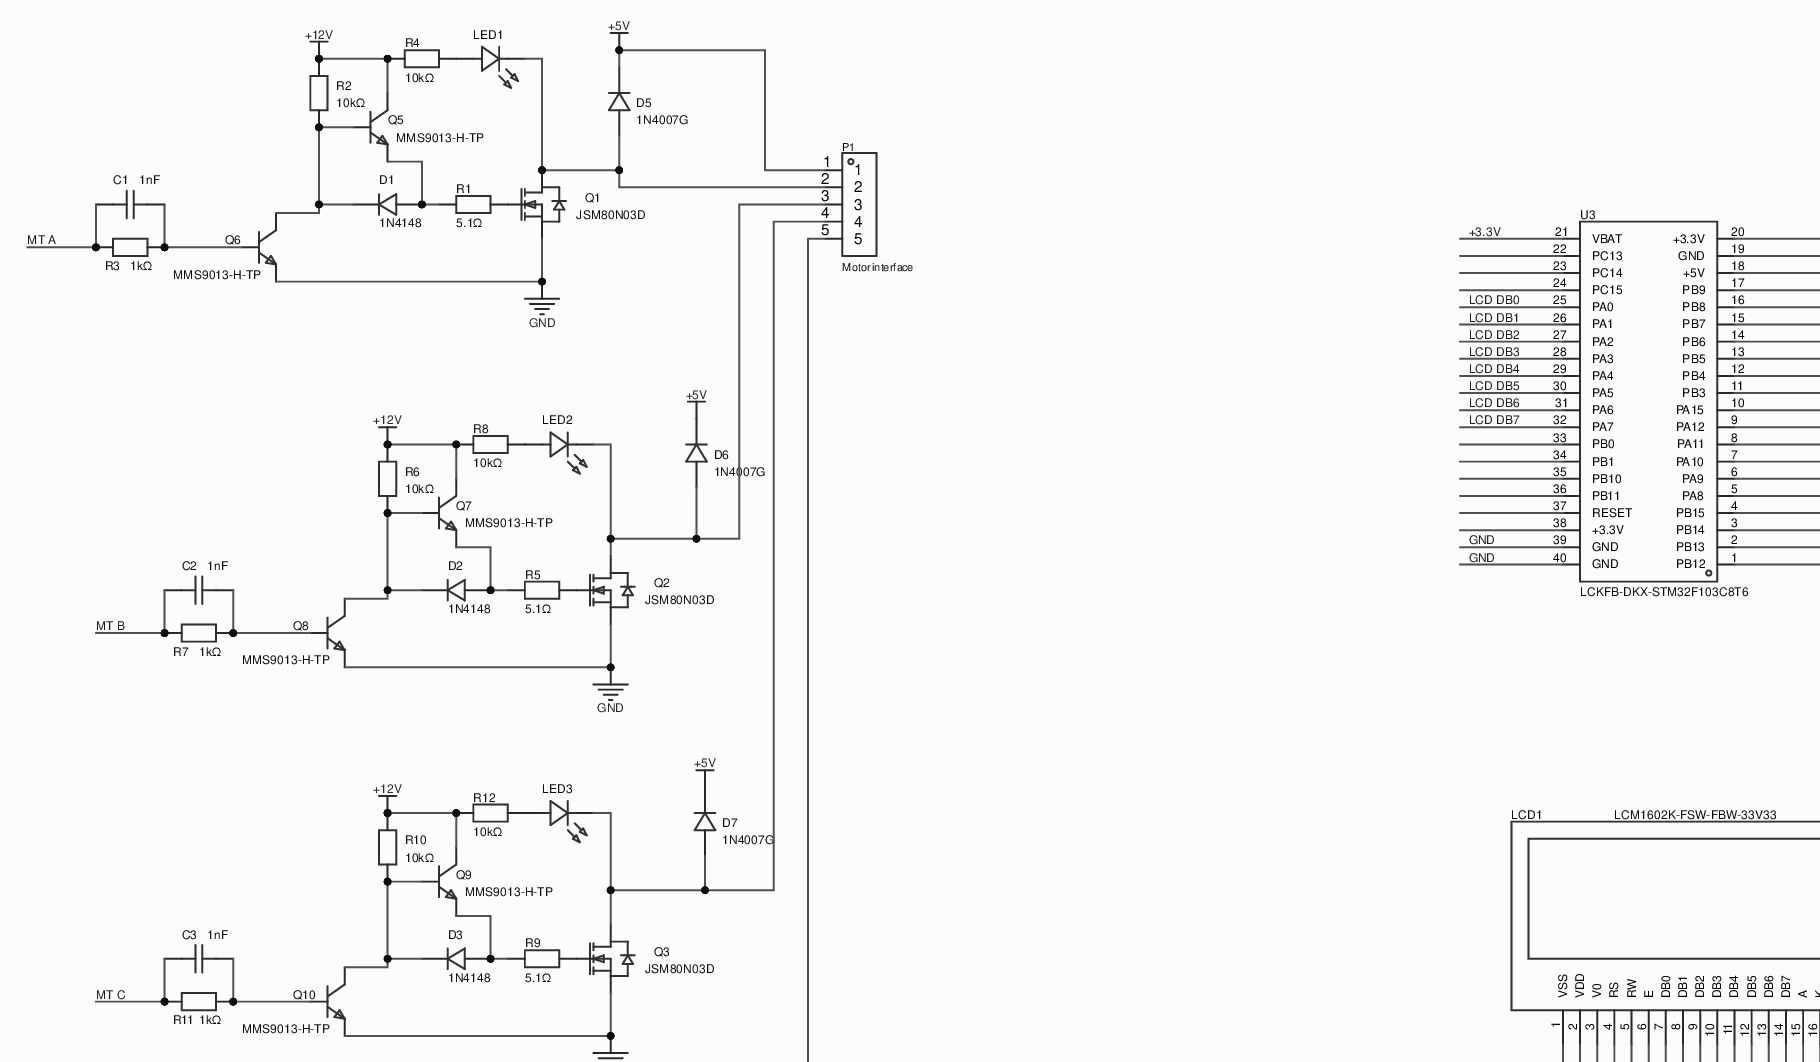
[diagram p0: MISC49935-3.schdoc, top left]
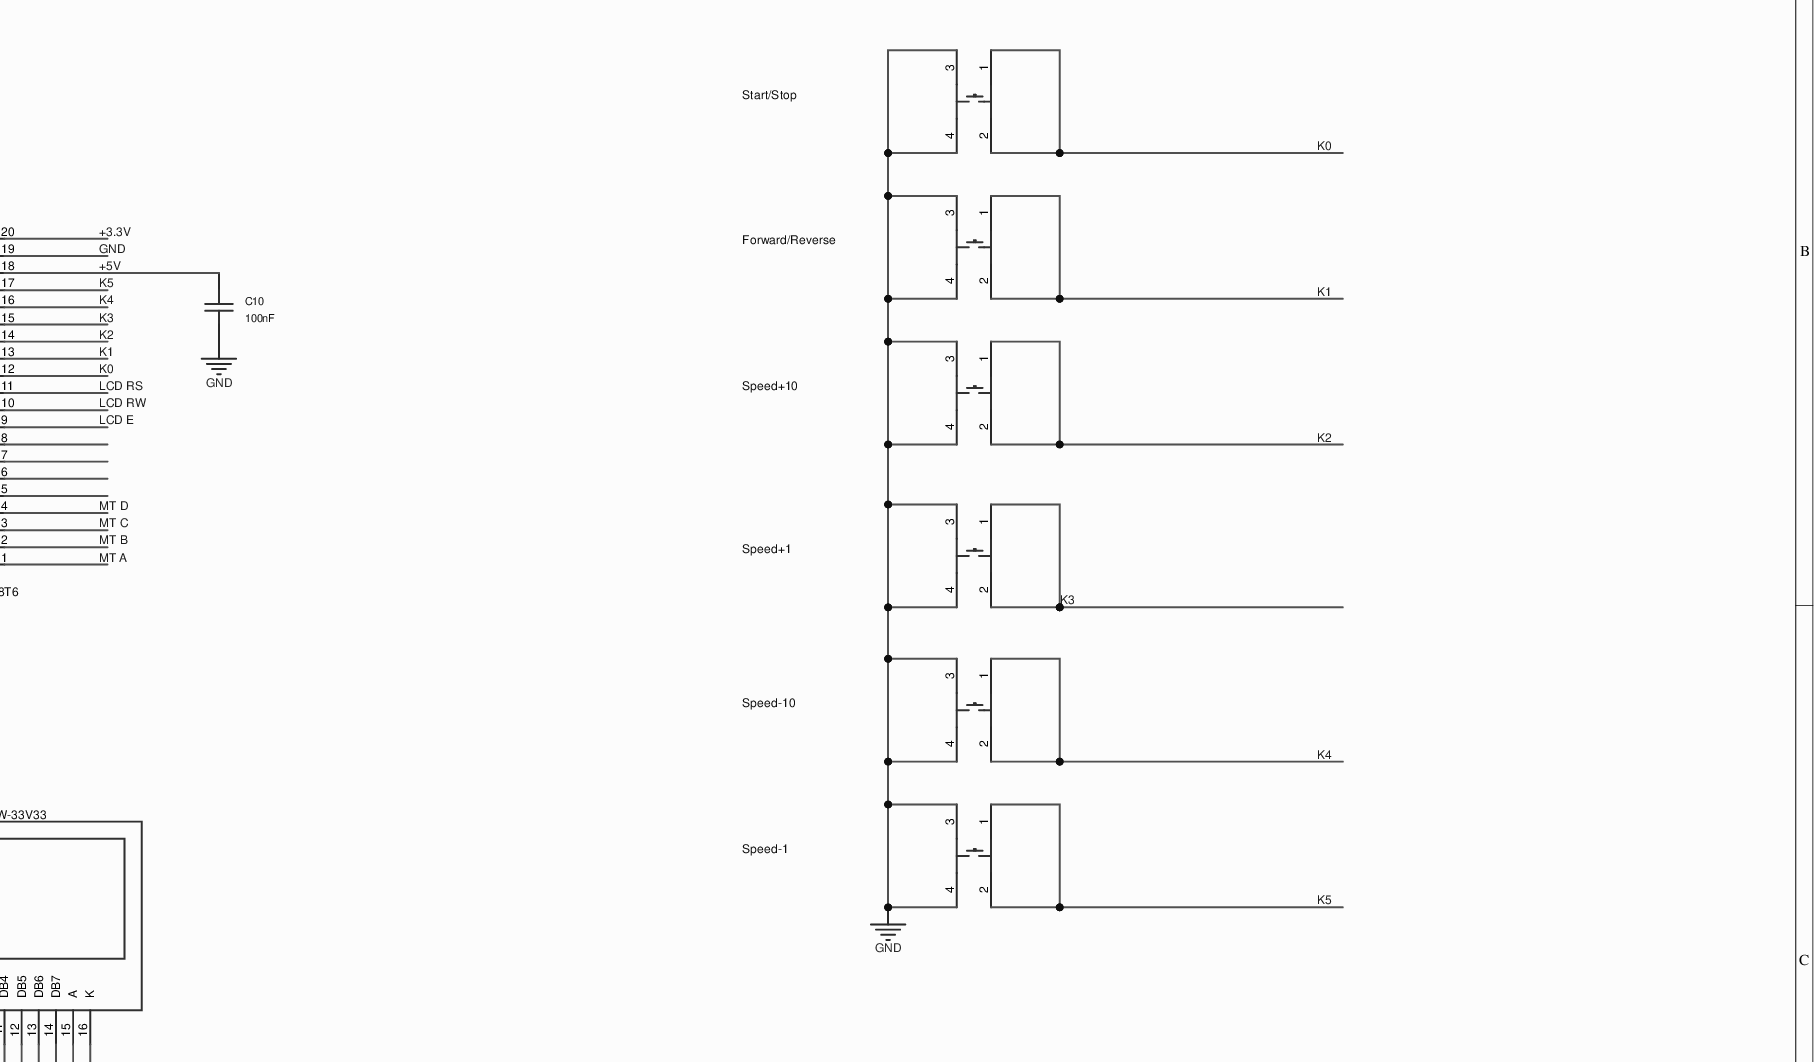
[diagram p1: MISC49935-3.schdoc, top right]
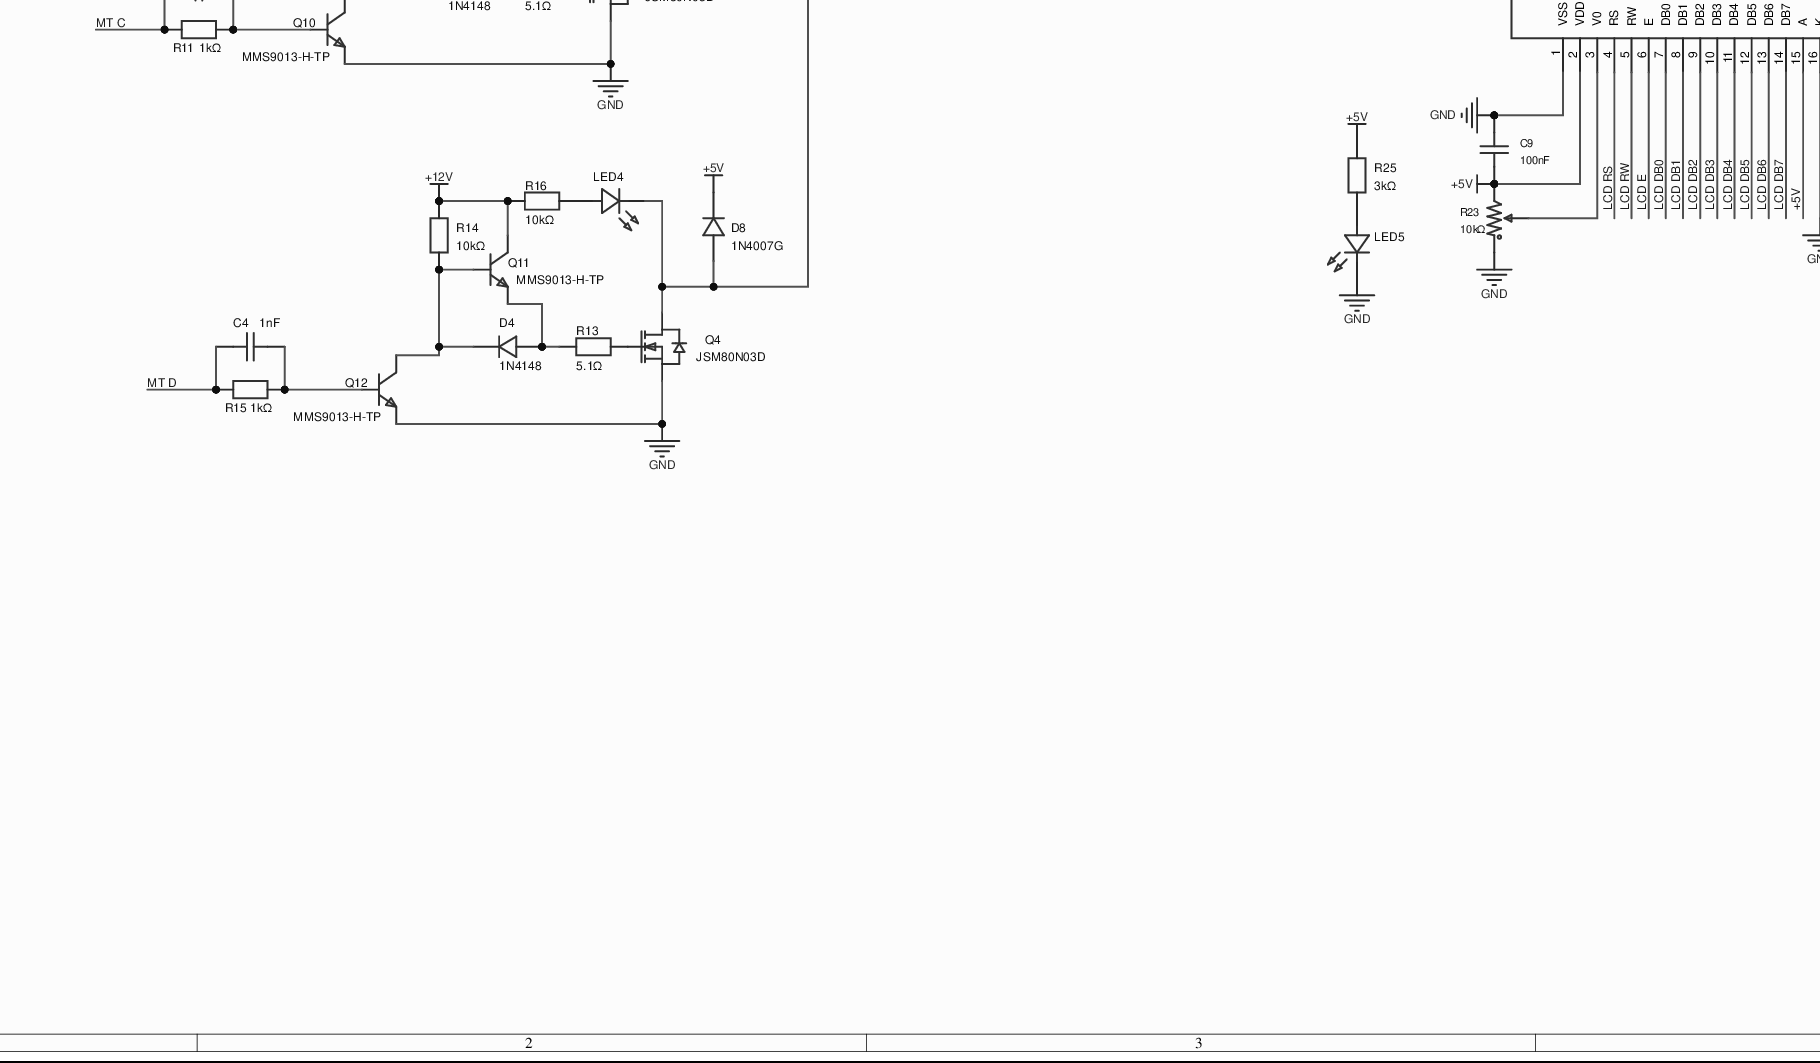
[diagram p2: MISC49935-3.schdoc, bottom left]
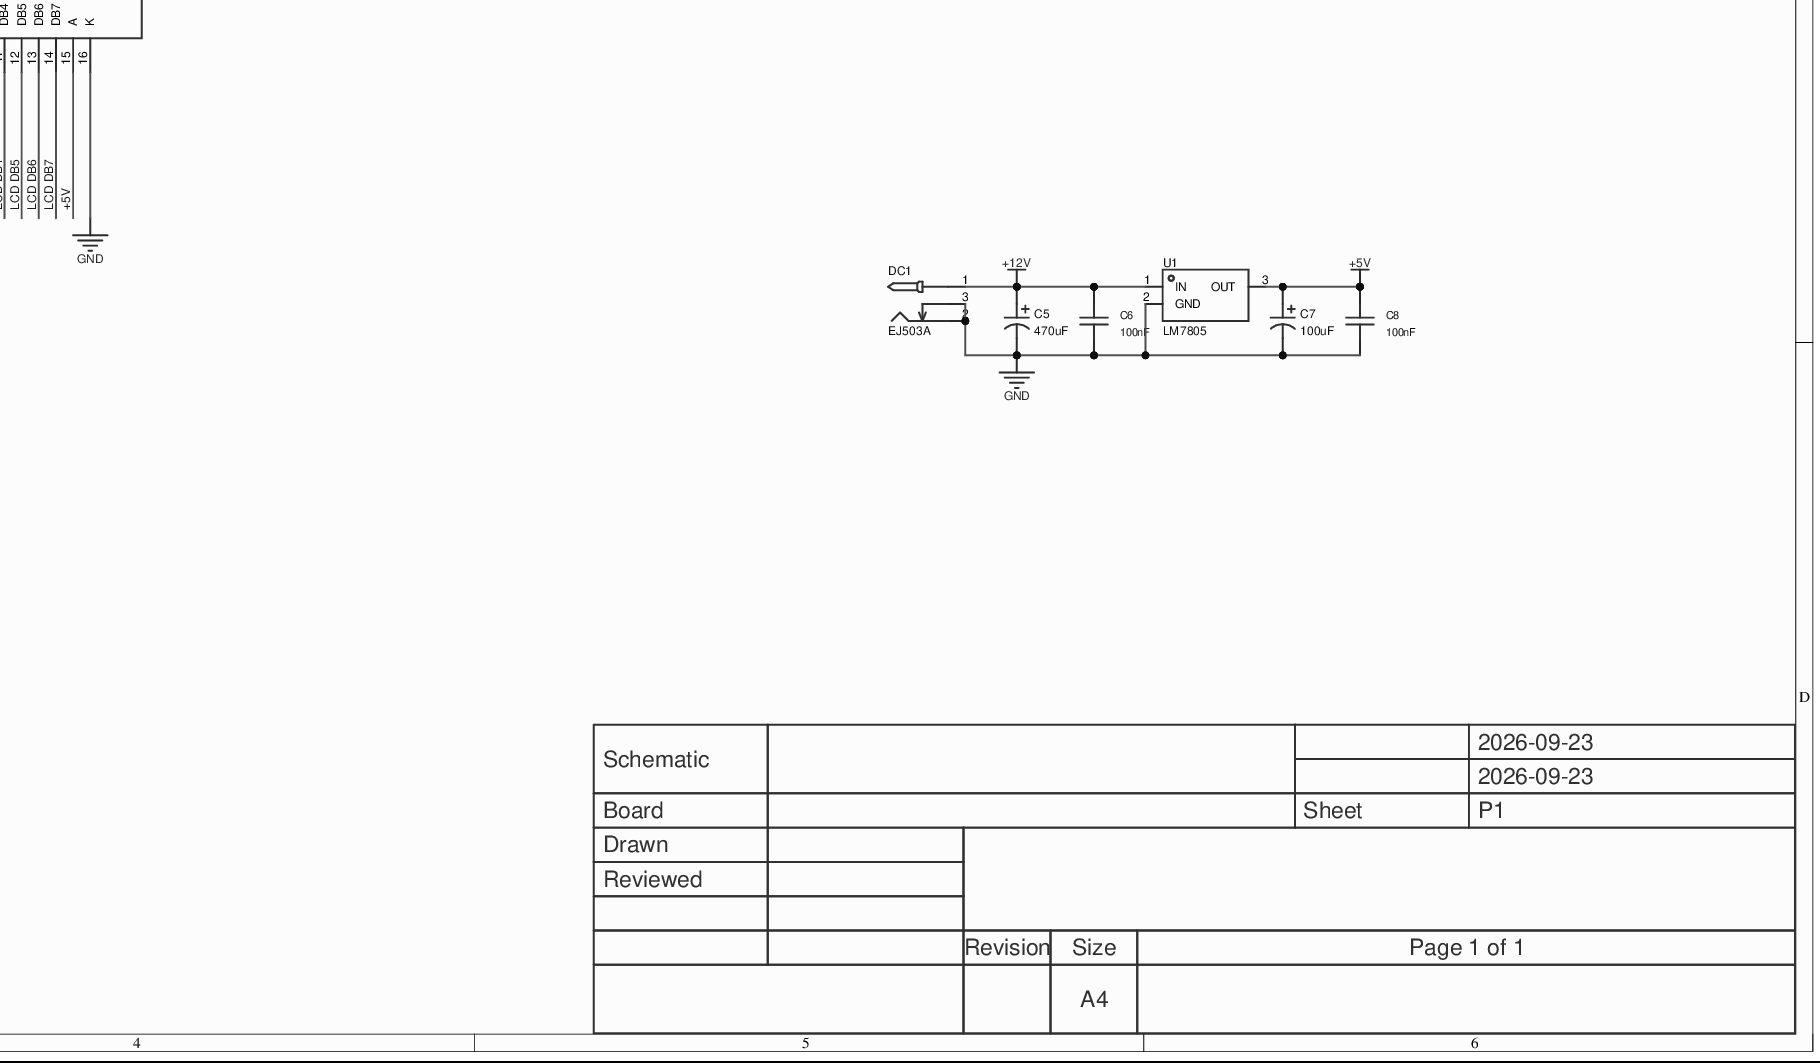
[diagram p3: MISC49935-3.schdoc, bottom right]
# Altium project MISC49935-2.PrjPcb
1 sheet, 64 parts. Net scope: global (net labels, ports and power ports of the same name join across sheets).
Board file: MISC49935.pcbdoc

## Sheet MISC49935-3.schdoc
size 594 x 420 mm; Name: MISC49935

### Parts
C1  1nF
C2  1nF
C3  1nF
C4  1nF
C5  470uF
C6  100nF
C7  100uF
C8  100nF
C9  100nF
C10  100nF
D1  1N4148
D2  1N4148
D3  1N4148
D4  1N4148
D5  1N4007G
D6  1N4007G
D7  1N4007G
D8  1N4007G
DC1  EJ503A
K0  Start/Stop
K1  Forward/Reverse
K2  Speed+10
K3  Speed+1
K4  Speed-10
K5  Speed-1
LCD1  LCM1602K-FSW-FBW-33V33
LED1  3mmFIR  (value not drawn)
LED2  3mmFIR  (value not drawn)
LED3  3mmFIR  (value not drawn)
LED4  3mmFIR  (value not drawn)
LED5  3mmFIR  (value not drawn)
P1  Motor interface
Q1  JSM80N03D
Q2  JSM80N03D
Q3  JSM80N03D
Q4  JSM80N03D
Q5  MMS9013-H-TP
Q6  MMS9013-H-TP
Q7  MMS9013-H-TP
Q8  MMS9013-H-TP
Q9  MMS9013-H-TP
Q10  MMS9013-H-TP
Q11  MMS9013-H-TP
Q12  MMS9013-H-TP
R1  5.1Ω  [R0603]
R2  10kΩ
R3  1kΩ
R4  10kΩ
R5  5.1Ω  [R0603]
R6  10kΩ
R7  1kΩ
R8  10kΩ
R9  5.1Ω  [R0603]
R10  10kΩ
R11  1kΩ
R12  10kΩ
R13  5.1Ω  [R0603]
R14  10kΩ
R15  1kΩ
R16  10kΩ
R23  10kΩ
R25  3kΩ
U1  LM7805
U3  LCKFB-DKX-STM32F103C8T6  [CONN-TH_L53.3-W22.9_STM32F103C8T6-CARD]

### Nets
+5V: C7.1 C8.2 C9.2 C10.1 D5.1(C) D6.1(C) D7.1(C) D8.1(C) LCD1.2(VDD) LCD1.15(A) P1.1 R23.3 R25.2 U1.3(OUT) U3.18(+5V)
+12V: C5.1 C6.2 DC1.1 Q5.3(C) Q7.3(C) Q9.3(C) Q11.3(C) R2.2 R4.1 R6.2 R8.1 R10.2 R12.1 R14.2 R16.1 U1.1(IN)
GND: C5.2 C6.1 C7.2 C8.1 C9.1 C10.2 DC1.2 DC1.3 K0.3 K0.4 K1.3 K1.4 K2.3 K2.4 K3.3 K3.4 K4.3 K4.4 K5.3 K5.4 LCD1.1(VSS) LCD1.16(K) LED5.2(K) Q1.3(S) Q2.3(S) Q3.3(S) Q4.3(S) Q6.2(E) Q8.2(E) Q10.2(E) Q12.2(E) R23.1 U1.2(GND) U3.19(GND) U3.39(GND) U3.40(GND)
+3.3V: U3.20(+3.3V) U3.21(VBAT)
K0: K0.1 K0.2 U3.12(PB4)
K1: K1.1 K1.2 U3.13(PB5)
K2: K2.1 K2.2 U3.14(PB6)
K3: K3.1 K3.2 U3.15(PB7)
K4: K4.1 K4.2 U3.16(PB8)
K5: K5.1 K5.2 U3.17(PB9)
LCD DB0: LCD1.7(DB0) U3.25(PA0)
LCD DB1: LCD1.8(DB1) U3.26(PA1)
LCD DB2: LCD1.9(DB2) U3.27(PA2)
LCD DB3: LCD1.10(DB3) U3.28(PA3)
LCD DB4: LCD1.11(DB4) U3.29(PA4)
LCD DB5: LCD1.12(DB5) U3.30(PA5)
LCD DB6: LCD1.13(DB6) U3.31(PA6)
LCD DB7: LCD1.14(DB7) U3.32(PA7)
LCD E: LCD1.6(E) U3.9(PA12)
LCD RS: LCD1.4(RS) U3.11(PB3)
LCD RW: LCD1.5(RW) U3.10(PA15)
MT A: C1.1 R3.1 U3.1(PB12)
MT B: C2.1 R7.1 U3.2(PB13)
MT C: C3.1 R11.1 U3.3(PB14)
MT D: C4.1 R15.1 U3.4(PB15)
NetC1_2: C1.2 Q6.1(B) R3.2
NetC2_2: C2.2 Q8.1(B) R7.2
NetC3_2: C3.2 Q10.1(B) R11.2
NetC4_2: C4.2 Q12.1(B) R15.2
NetD1_1: D1.1(A) Q5.2(E) R1.1
NetD1_2: D1.2(C) Q5.1(B) Q6.3(C) R2.1
NetD2_1: D2.1(A) Q7.2(E) R5.1
NetD2_2: D2.2(C) Q7.1(B) Q8.3(C) R6.1
NetD3_1: D3.1(A) Q9.2(E) R9.1
NetD3_2: D3.2(C) Q9.1(B) Q10.3(C) R10.1
NetD4_1: D4.1(A) Q11.2(E) R13.1
NetD4_2: D4.2(C) Q11.1(B) Q12.3(C) R14.1
NetD5_2: D5.2(A) LED1.2(K) P1.2 Q1.2(D)
NetD6_2: D6.2(A) LED2.2(K) P1.3 Q2.2(D)
NetD7_2: D7.2(A) LED3.2(K) P1.4 Q3.2(D)
NetD8_2: D8.2(A) LED4.2(K) P1.5 Q4.2(D)
NetLCD1_3: LCD1.3(V0) R23.2
NetLED1_1: LED1.1(A) R4.2
NetLED2_1: LED2.1(A) R8.2
NetLED3_1: LED3.1(A) R12.2
NetLED4_1: LED4.1(A) R16.2
NetLED5_1: LED5.1(A) R25.1
NetQ1_1: Q1.1(G) R1.2
NetQ2_1: Q2.1(G) R5.2
NetQ3_1: Q3.1(G) R9.2
NetQ4_1: Q4.1(G) R13.2

Not connected (* = marked no-connect by the designer): U3 5(PA8) 6(PA9) 7(PA10) 8(PA11) 22(PC13) 23(PC14) 24(PC15) 33(PB0) 34(PB1) 35(PB10) 36(PB11) 37(RESET) 38(+3.3V)

### Notes on the sheet
- 2026-09-23
- Schematic
- Board
- Sheet
- P1
- Drawn
- Reviewed
- Revision
- Size
- A4
- Page 1 of 1

### Library data of the parts
C1-C4 = KY1102M400VAC70Y10093: Capacitance: 1nF; tolerance: ±20%; working voltage (AC): 400V; protection class: Y1;; Manufacturer: KNSCHA(科尼盛); Add into BOM: yes; 3D Model: 9383b9b23f884ae7b98244ec8344dac50819f05c4eef4c71ace90d822a990e87; 3D Model Transform: 431.76158,177.165,0,0,0,0,0,0,-137.795; safety certification: UL; ENEC; VDE; CQC; Origin Footprint: CAP-TH_L7.5-W4.5-P10.00-D0.6; Device: KY1102M400VAC70Y10093; Symbol: KY1102M400VAC70Y10093; LCSC Part Name: 1nF ±20% 400V 等级:Y1; Supplier Part: C2943996; Manufacturer Part: KY1102M400VAC70Y10093; Supplier Footprint: 插件,P=10mm; JLCPCB Part Class: Extended Part; Datasheet: example.com/datasheet/KY1102M400VAC70Y10093/3329207.html; Supplier: LCSC; Convert to PCB: yes; Value: 1nF; Tolerance: ±20%; Voltage(AC): 400V; Ratings: Y1; ModelName: CAP-TH_L7.5-W4.5-P10.00-D0.6
C5 = JVJ35V470M10x10: Capacitance: 470uF; tolerance: ±20%; rated voltage: 35V; ripple current: 320mA@120Hz;; Manufacturer: JIERR(捷而瑞); Add into BOM: yes; 3D Model: 6492d35f87704f6c8eef04ed8ab17b430819f05c4eef4c71ace90d822a990e87; 3D Model Transform: 433.07,405.511,0,0,0,0,0,0,0; Lifetime: 2000hrs@105℃; Origin Footprint: CAP-SMD_BD10.0-L10.3-W10.3-LS11.0; Device: JVJ35V470M10x10; Symbol: JVJ35V470M10x10; LCSC Part Name: 470uF ±20% 35V; Supplier Part: C46550413; Manufacturer Part: JVJ35V470M10x10; Supplier Footprint: SMD,D10xL10.5mm; JLCPCB Part Class: Extended Part; Datasheet: example.com/datasheet/JVJ35V470M10x10/48680107.html; Supplier: LCSC; Convert to PCB: yes; Value: 470uF; Tolerance: ±20%; Voltage Rating: 35V; Ripple Current: 320mA@120Hz; Diameter: 10mm; Height - Seated (Max): 10.5mm; Operating Temperature: -55℃~+105℃; ModelName: CAP-SMD_BD10.0-L10.3-W10.3-LS11.0
C6 C8-C10 = MPE104J100V0501: Capacitance: 100nF; tolerance: ±5%; rated voltage: 100V; operating temperature: -55℃~+105℃;; Manufacturer: JIERR(捷而瑞); Add into BOM: yes; 3D Model: 2ff8eac0344a4af6b7779afed8020edb0819f05c4eef4c71ace90d822a990e87; 3D Model Transform: 248.031,118.5037,0,0,0,0,-0.005,0,-177.165; Origin Footprint: CAP-TH_L6.3-W3.0-P5.00-D0.5; Device: MPE104J100V0501; Symbol: MPE104J100V0501; LCSC Part Name: 100nF ±5% 100V; Supplier Part: C55219016; Manufacturer Part: MPE104J100V0501; Supplier Footprint: 插件,P=5mm; JLCPCB Part Class: Extended Part; Datasheet: example.com/datasheet/MPE104J100V0501/59064466.html; Supplier: LCSC; Convert to PCB: yes; Value: 100nF; Tolerance: ±5%; Voltage Rating: 100V; Operating Temperature: -55℃~+105℃; ModelName: CAP-TH_L6.3-W3.0-P5.00-D0.5
C7 = JVJ50V100M6x8: Capacitance: 100uF; tolerance: ±20%; rated voltage: 50V; ripple current: 140mA@120Hz;; Manufacturer: JIERR(捷而瑞); Add into BOM: yes; 3D Model: ccbda52dceed4b139172c40f75c9da3f0819f05c4eef4c71ace90d822a990e87; 3D Model Transform: 287.401,259.842,0,0,0,0,0,0,0; Lifetime: 2000hrs@105℃; Origin Footprint: CAP-SMD_BD6.3-L6.6-W6.6-LS7.3-FD-H7.7; Device: JVJ50V100M6x8; Symbol: JVJ50V100M6x8; LCSC Part Name: 100uF ±20% 50V; Supplier Part: C46550415; Manufacturer Part: JVJ50V100M6x8; Supplier Footprint: SMD,D6.3xL7.7mm; JLCPCB Part Class: Extended Part; Datasheet: example.com/datasheet/JVJ50V100M6x8/48680109.html; Supplier: LCSC; Convert to PCB: yes; Value: 100uF; Tolerance: ±20%; Voltage Rating: 50V; Ripple Current: 140mA@120Hz; Diameter: 6.3mm; Height - Seated (Max): 7.7mm; Operating Temperature: -55℃~+105℃; ModelName: CAP-SMD_BD6.3-L6.6-W6.6-LS7.3-FD-H7.7
D1-D4 = 1N4148_C9900036548: Add into BOM: yes; 3D Model: b29439ed7b924f62acded4384188502f0819f05c4eef4c71ace90d822a990e87; 3D Model Transform: 334.645,87.008,0,0,0,0,0,0,-196.85; Origin Footprint: DO-35_BD2.2-L4.0-D0.50_1N4148; Device: 1N4148_C9900036548; Symbol: 1N4148_C9900036548; LCSC Part Name: 1N4148; Supplier Part: C9900036548; Manufacturer Part: 1N4148; Supplier Footprint: LL34; JLCPCB Part Class: Extended Part; Supplier: LCSC; Convert to PCB: yes; ModelName: DO-35_BD2.2-L4.0-D0.50_1N4148
D5-D8 = 1N4007G_C2457: Diode configuration: 1 discrete; forward voltage (Vf): 1.1V@1A; reverse voltage (Vr): 1kV; rectified current: 1A;; Manufacturer: MDD(辰达半导体); Add into BOM: yes; 3D Model: 6de1e9b71a0d4751b4e9df530304c1a30819f05c4eef4c71ace90d822a990e87; 3D Model Transform: 374.016,94.488,0,0,0,0,0,0,-137.795; Reverse Leakage Current (Ir): 5uA@1kV; Non-Repetitive Peak Forward Surge Current: 30A; Operating Junction Temperature Range: -65℃~+150℃; Origin Footprint: DO-41_BD2.4-L4.7-P8.70-D0.9-RD; ModelName: DO-41_D2.4-L4.7-P8.70; Device: 1N4007G_C2457; Symbol: 1N4007G_C2457; LCSC Part Name: 1kV 1A; Supplier Part: C2457; Manufacturer Part: 1N4007G; Supplier Footprint: DO-41; JLCPCB Part Class: Extended Part; Datasheet: example.com/datasheet/1N4007G/2834.html; Supplier: LCSC; Convert to PCB: yes; Diode Configuration: 1 discrete; Voltage - Forward(Vf@If): 1.1V@1A; Voltage - DC Reverse(Vr): 1kV; Current - Rectified: 1A
DC1 = EJ503A: Connector type: DC power jack; mounting: right-angle through-hole; contact inner diameter: 2.1mm; contact outer diameter: 5.5mm; rated current: 5A; rated voltage: 12V; operating temperature: -15℃~+90℃;; Manufacturer: MPD(Memory Protection Devices); Add into BOM: yes; 3D Model: 9b2360b4158442638544318d1240cc000819f05c4eef4c71ace90d822a990e87; 3D Model Transform: 369.2906,575.589,0,0,0,0,-83.66,-140.747,-169.291; Body Height: 11mm; Origin Footprint: DC-IN-TH_EJ503A; Device: EJ503A; Symbol: EJ503A; LCSC Part Name: DC电源插座 内径:2.1mm 外径:5.5mm; Supplier Part: C3095117; Manufacturer Part: EJ503A; Supplier Footprint: 插件; JLCPCB Part Class: Extended Part; Datasheet: example.com/datasheet/EJ503A/3654351.html; Supplier: LCSC; Convert to PCB: yes; Connector Type: DC power jack; Mounting Type: Right-angle through-hole; Inside Contact Diameter: 2.1mm; Outside Contact Diameter: 5.5mm; Current Rating: 5A; Voltage Rating (Max): 12V; Length: 13.7mm; Width: 9mm; Operating Temperature: -15℃~+90℃; ModelName: DC-IN-TH_EJ503A
K0 = TS-1002S-04526C_1: Circuit: SPST; button shape: round button; actuating force: 2.6N; mounting: upright SMD; switch length: 6mm; switch width: 6mm; switch height: 4.5mm; bracket: without bracket; contact current: 50mA; rated voltage: 12V; LED: -; operating life: -;; Manufacturer: XUNPU(讯普); Add into BOM: yes; 3D Model: fbf4ceca6c4742d48614ab6a891ef9810819f05c4eef4c71ace90d822a990e87; 3D Model Transform: 330.708,251.968,0,0,0,0,0,-0.005,0; Actuator/Cap Color: Black; Origin Footprint: SW-SMD_4P-L6.0-W6.0-P4.50-LS9.0-2; Device: TS-1002S-04526C_1; Symbol: TS-1002S-04526C; LCSC Part Name: 6*6*4.5mm 立贴 轻触开关; Supplier Part: C455109; Manufacturer Part: TS-1002S-04526C; Supplier Footprint: SMD-4P,6x6mm; JLCPCB Part Class: Extended Part; Datasheet: example.com/datasheet/TS-1002S-04526C/457514.html; Supplier: LCSC; Convert to PCB: yes; Actuator Style: Round button; Operating Force: 2.6N; Mounting Type: Upright SMD; Length: 6mm; Width: 6mm; Switch Height: 4.5mm; with Bracket: Without bracket; Contact Current: 50mA; Voltage Rating: 12V; With Lamp: -; Termination Style: Gull-wing; Life: -
K1 = TS-1002S-04526C: Circuit: SPST; button shape: round button; actuating force: 2.6N; mounting: upright SMD; switch length: 6mm; switch width: 6mm; switch height: 4.5mm; bracket: without bracket; contact current: 50mA; rated voltage: 12V; LED: -; operating life: -;; Manufacturer: XUNPU(讯普); Add into BOM: yes; 3D Model: fbf4ceca6c4742d48614ab6a891ef9810819f05c4eef4c71ace90d822a990e87; 3D Model Transform: 330.708,251.968,0,0,0,0,0,-0.005,0; Actuator/Cap Color: Black; Origin Footprint: SW-SMD_4P-L6.0-W6.0-P4.50-LS9.0-2; Device: TS-1002S-04526C; Symbol: TS-1002S-04526C; LCSC Part Name: 6*6*4.5mm 立贴 轻触开关; Supplier Part: C455109; Manufacturer Part: TS-1002S-04526C; Supplier Footprint: SMD-4P,6x6mm; JLCPCB Part Class: Extended Part; Datasheet: example.com/datasheet/TS-1002S-04526C/457514.html; Supplier: LCSC; Convert to PCB: yes; Actuator Style: Round button; Operating Force: 2.6N; Mounting Type: Upright SMD; Length: 6mm; Width: 6mm; Switch Height: 4.5mm; with Bracket: Without bracket; Contact Current: 50mA; Voltage Rating: 12V; With Lamp: -; Termination Style: Gull-wing; Life: -
K2 = TS-1002S-04526C_4: Circuit: SPST; button shape: round button; actuating force: 2.6N; mounting: upright SMD; switch length: 6mm; switch width: 6mm; switch height: 4.5mm; bracket: without bracket; contact current: 50mA; rated voltage: 12V; LED: -; operating life: -;; Manufacturer: XUNPU(讯普); Add into BOM: yes; 3D Model: fbf4ceca6c4742d48614ab6a891ef9810819f05c4eef4c71ace90d822a990e87; 3D Model Transform: 330.708,251.968,0,0,0,0,0,-0.005,0; Actuator/Cap Color: Black; Origin Footprint: SW-SMD_4P-L6.0-W6.0-P4.50-LS9.0-2; Device: TS-1002S-04526C_4; Symbol: TS-1002S-04526C; LCSC Part Name: 6*6*4.5mm 立贴 轻触开关; Supplier Part: C455109; Manufacturer Part: TS-1002S-04526C; Supplier Footprint: SMD-4P,6x6mm; JLCPCB Part Class: Extended Part; Datasheet: example.com/datasheet/TS-1002S-04526C/457514.html; Supplier: LCSC; Convert to PCB: yes; Actuator Style: Round button; Operating Force: 2.6N; Mounting Type: Upright SMD; Length: 6mm; Width: 6mm; Switch Height: 4.5mm; with Bracket: Without bracket; Contact Current: 50mA; Voltage Rating: 12V; With Lamp: -; Termination Style: Gull-wing; Life: -
K3 = TS-1002S-04526C_2: Circuit: SPST; button shape: round button; actuating force: 2.6N; mounting: upright SMD; switch length: 6mm; switch width: 6mm; switch height: 4.5mm; bracket: without bracket; contact current: 50mA; rated voltage: 12V; LED: -; operating life: -;; Manufacturer: XUNPU(讯普); Add into BOM: yes; 3D Model: fbf4ceca6c4742d48614ab6a891ef9810819f05c4eef4c71ace90d822a990e87; 3D Model Transform: 330.708,251.968,0,0,0,0,0,-0.005,0; Actuator/Cap Color: Black; Origin Footprint: SW-SMD_4P-L6.0-W6.0-P4.50-LS9.0-2; Device: TS-1002S-04526C_2; Symbol: TS-1002S-04526C; LCSC Part Name: 6*6*4.5mm 立贴 轻触开关; Supplier Part: C455109; Manufacturer Part: TS-1002S-04526C; Supplier Footprint: SMD-4P,6x6mm; JLCPCB Part Class: Extended Part; Datasheet: example.com/datasheet/TS-1002S-04526C/457514.html; Supplier: LCSC; Convert to PCB: yes; Actuator Style: Round button; Operating Force: 2.6N; Mounting Type: Upright SMD; Length: 6mm; Width: 6mm; Switch Height: 4.5mm; with Bracket: Without bracket; Contact Current: 50mA; Voltage Rating: 12V; With Lamp: -; Termination Style: Gull-wing; Life: -
K4 = TS-1002S-04526C_5: Circuit: SPST; button shape: round button; actuating force: 2.6N; mounting: upright SMD; switch length: 6mm; switch width: 6mm; switch height: 4.5mm; bracket: without bracket; contact current: 50mA; rated voltage: 12V; LED: -; operating life: -;; Manufacturer: XUNPU(讯普); Add into BOM: yes; 3D Model: fbf4ceca6c4742d48614ab6a891ef9810819f05c4eef4c71ace90d822a990e87; 3D Model Transform: 330.708,251.968,0,0,0,0,0,-0.005,0; Actuator/Cap Color: Black; Origin Footprint: SW-SMD_4P-L6.0-W6.0-P4.50-LS9.0-2; Device: TS-1002S-04526C_5; Symbol: TS-1002S-04526C; LCSC Part Name: 6*6*4.5mm 立贴 轻触开关; Supplier Part: C455109; Manufacturer Part: TS-1002S-04526C; Supplier Footprint: SMD-4P,6x6mm; JLCPCB Part Class: Extended Part; Datasheet: example.com/datasheet/TS-1002S-04526C/457514.html; Supplier: LCSC; Convert to PCB: yes; Actuator Style: Round button; Operating Force: 2.6N; Mounting Type: Upright SMD; Length: 6mm; Width: 6mm; Switch Height: 4.5mm; with Bracket: Without bracket; Contact Current: 50mA; Voltage Rating: 12V; With Lamp: -; Termination Style: Gull-wing; Life: -
K5 = TS-1002S-04526C_3: Circuit: SPST; button shape: round button; actuating force: 2.6N; mounting: upright SMD; switch length: 6mm; switch width: 6mm; switch height: 4.5mm; bracket: without bracket; contact current: 50mA; rated voltage: 12V; LED: -; operating life: -;; Manufacturer: XUNPU(讯普); Add into BOM: yes; 3D Model: fbf4ceca6c4742d48614ab6a891ef9810819f05c4eef4c71ace90d822a990e87; 3D Model Transform: 330.708,251.968,0,0,0,0,0,-0.005,0; Actuator/Cap Color: Black; Origin Footprint: SW-SMD_4P-L6.0-W6.0-P4.50-LS9.0-2; Device: TS-1002S-04526C_3; Symbol: TS-1002S-04526C; LCSC Part Name: 6*6*4.5mm 立贴 轻触开关; Supplier Part: C455109; Manufacturer Part: TS-1002S-04526C; Supplier Footprint: SMD-4P,6x6mm; JLCPCB Part Class: Extended Part; Datasheet: example.com/datasheet/TS-1002S-04526C/457514.html; Supplier: LCSC; Convert to PCB: yes; Actuator Style: Round button; Operating Force: 2.6N; Mounting Type: Upright SMD; Length: 6mm; Width: 6mm; Switch Height: 4.5mm; with Bracket: Without bracket; Contact Current: 50mA; Voltage Rating: 12V; With Lamp: -; Termination Style: Gull-wing; Life: -
LCD1 = LCM1602K-FSW-FBW-33V33: Controller chip: KS0066U; size (inch): -;; Manufacturer: LONTECH(厦门龙特); Add into BOM: yes; 3D Model: 84dc4c036e12490da40aa0593fb5d02d0819f05c4eef4c71ace90d822a990e87; 3D Model Transform: 3149.6,1417.32,0,0,0,0,509.803,-610.157,0; Origin Footprint: MODULE-TH_LCM1602K; Device: LCM1602K-FSW-FBW-33V33; Symbol: LCM1602K-FSW-FBW-33V33; LCSC Part Name: LCM1602K-FSW-FBW-33V33; Supplier Part: C83271; Manufacturer Part: LCM1602K-FSW-FBW-33V33; Supplier Footprint: -; JLCPCB Part Class: Extended Part; Datasheet: example.com/upload/public/pdf/source/20161111/1478835367700.pdf; Supplier: LCSC; Convert to PCB: yes; Main Control Chip: KS0066U; Size: -; ModelName: MODULE-TH_LCM1602K
LED1-LED5 = 3mmFIR: Add into BOM: yes; 3D Model: a497c992633541038a38947cdc58012f0819f05c4eef4c71ace90d822a990e87; 3D Model Transform: 141.274,153.327,0,0,0,0,-5.984,0,-137.795; Origin Footprint: LED-TH_BD3.0-P2.54-FD; Device: 3mmFIR; Symbol: 3mmFIR; LCSC Part Name: 3mmFIR; Supplier Part: C9900095018; Manufacturer Part: 3mmFIR; Supplier Footprint: LED-TH_LED-3MM_RED; JLCPCB Part Class: Extended Part; Supplier: LCSC; Convert to PCB: yes
P1 = LAIL-PZ2.54-5P-L: Pin structure: 1x5P; pitch: 2.54mm; pin type: square; rows: single row; total pins: 5P; rated current: 3A; rated voltage: 250V; insulator height: 2.5mm; end pin length: 3mm; contact material: brass; contact plating: gold; operating temperature: -25℃~+80℃; colour: black;; Manufacturer: LAILAN(莱联); Add into BOM: yes; 3D Model: e1dcc648b849411f93f4e3449eac68780819f05c4eef4c71ace90d822a990e87; 3D Model Transform: 499.999,98.8187,0,0,0,0,0,0,-118.11; Origin Footprint: CONN-TH_LAIL-PZ2.54-5P-L; Device: LAIL-PZ2.54-5P-L; Symbol: LAIL-PZ2.54-5P-L; LCSC Part Name: 1x5P 间距:2.54mm 方针; Supplier Part: C54950605; Manufacturer Part: LAIL-PZ2.54-5P-L; Supplier Footprint: 插件,P=2.54mm; JLCPCB Part Class: Extended Part; Datasheet: example.com/datasheet/LAIL-PZ2.54-5P-L/58519958.html; Supplier: LCSC; Convert to PCB: yes; Pin Structure: 1x5P; Pitch: 2.54mm; Circluar Pins/Square Pins: Square; Number of Rows: Single row; Number of Pins: 5P; Current Rating: 3A; Voltage Rating (Max): 250V; Insulation Height: 2.5mm; Length of End Connection Pin: 3mm; Contact Material: Brass; Contact Plating: Gold; Operating Temperature: -25℃~+80℃; Color: Black; ModelName: CONN-TH_LAIL-PZ2.54-5P-L
Q1-Q4 = JSM80N03D: Quantity: 1 N-channel; drain-source voltage (Vdss): 30V; continuous drain current (Id): 80A; on-resistance (RDS(on)): 7.5mΩ@4.5V; 4.2mΩ@10V; power dissipation (Pd): 46W; threshold voltage (Vgs(th)): 1.5V;; Manufacturer: JSMSEMI(杰盛微); Add into BOM: yes; 3D Model: ce57f84d66384067af8a68020b6de06d0819f05c4eef4c71ace90d822a990e87; 3D Model Transform: 259.842,390.52442,0,90,0,0,-39.39,0,0; Gate Charge(Qg): 33.7nC@10V; Input Capacitance(Ciss): 1.614nF; Reverse Transfer Capacitance (Crss@Vds): 215pF; Output Capacitance(Coss): 245pF; Origin Footprint: TO-252-2_L6.6-W6.1-P4.57-LS9.9-BR-CW; Device: JSM80N03D; Symbol: JSM80N03D; LCSC Part Name: N沟道 30V 80A; Supplier Part: C22447118; Manufacturer Part: JSM80N03D; Supplier Footprint: TO-252; JLCPCB Part Class: Extended Part; Datasheet: example.com/datasheet/JSM80N03D/24102040.html; Supplier: LCSC; Convert to PCB: yes; Number: 1 N-channel; Drain to Source Voltage: 30V; Current - Continuous Drain(Id): 80A; RDS(on): 7.5mΩ@4.5V; 4.2mΩ@10V; Pd - Power Dissipation: 46W; Gate Threshold Voltage (Vgs(th)): 1.5V; Operating Temperature: -55℃~+150℃; Type: N-channel
Q5-Q12 = MMS9013-H-TP: Transistor type: NPN; collector current (Ic): 500mA; collector-emitter breakdown voltage (Vceo): 25V; power dissipation (Pd): 300mW; DC current gain (hFE): 350;; Manufacturer: MCC(美微科); Add into BOM: yes; 3D Model: c62791f0466c4ae2a892c056b845b0ca0819f05c4eef4c71ace90d822a990e87; 3D Model Transform: 98.425,114.173,0,180,0,0,0.0005,-0.0005,0; DC Current Gain: 350; Transition frequency(fT): 150MHz; Current - Collector Cutoff: 100nA; Vce Saturation(VCE(sat)): 600mV; Emitter-Base Voltage(Vebo): 5V; Number: 1 NPN; Origin Footprint: SOT-23-3_L2.9-W1.3-P1.90-LS2.4-BR; Device: MMS9013-H-TP; Symbol: MMS9013-H-TP; LCSC Part Name: NPN 电流:500mA 电压:25V; Supplier Part: C90160; Manufacturer Part: MMS9013-H-TP; Supplier Footprint: SOT-23; JLCPCB Part Class: Extended Part; Datasheet: example.com/datasheet/MMS9013-H-TP/91345.html; Supplier: LCSC; Convert to PCB: yes; type: NPN; Current - Collector(Ic): 500mA; Collector - Emitter Voltage VCEO: 25V; Pd - Power Dissipation: 300mW; Operating Temperature: -55℃~+150℃
R1 R5 R9 R13 = FRC0603F5R10TS: Resistor type: thick film resistor; resistance: 5.1Ω; tolerance: ±1%; power: 100mW; working voltage: 75V; temperature coefficient: ±200ppm/℃;; Manufacturer: FOJAN(富捷); Add into BOM: yes; 3D Model: fc143cca1e79419f9cd78b61e9279f080819f05c4eef4c71ace90d822a990e87; 3D Model Transform: 31.8897,63.7794,0,90,0,0,0,0,0; Device: FRC0603F5R10TS; Symbol: FRC0603F5R10TS; LCSC Part Name: 5.1Ω ±1% 100mW 厚膜电阻; Supplier Part: C2907045; Manufacturer Part: FRC0603F5R10TS; Supplier Footprint: 0603; JLCPCB Part Class: Extended Part; Supplier: LCSC; Convert to PCB: yes; Type: Thick film resistor; Value: 5.1Ω; Tolerance: ±1%; Power(Watts): 100mW; Voltage-Supply(Max): 75V; Temperature Coefficient: ±200ppm/℃; Operating Temperature: -55℃~+155℃; Origin Footprint: R0603; FootprintName: R0603; ModelName: R0603
R2 R6 R10 R14 = MGR02WJ0103A10: Resistor type: carbon film resistor; resistance: 10kΩ; tolerance: ±5%; power: 2W; temperature coefficient: ±200ppm/℃;; Manufacturer: UNI-ROYAL(厚声); Add into BOM: yes; 3D Model: 603910ed2f70472a83476a25508c39d90819f05c4eef4c71ace90d822a990e87; 3D Model Transform: 795.27392,196.25953,0,0,0,0,0,0,-196.85; Origin Footprint: RES-TH_BD5.0-L15.5-P19.50-D0.7; Device: MGR02WJ0103A10; Symbol: MGR02WJ0103A10; LCSC Part Name: MGR02WJ0103A10; Supplier Part: C30187422; Manufacturer Part: MGR02WJ0103A10; Supplier Footprint: 插件,D5xL15.5mm; Datasheet: example.com/datasheet/MGR02WJ0103A10/31922950.html; Supplier: LCSC; Convert to PCB: yes; Type: Carbon film resistor; Value: 10kΩ; Tolerance: ±5%; Power(Watts): 2W; Temperature Coefficient: ±200ppm/℃
R3 R7 R11 R15 = MGR02WJ0102A10: Resistor type: carbon film resistor; resistance: 1kΩ; tolerance: ±5%; power: 2W;; Manufacturer: UNI-ROYAL(厚声); Add into BOM: yes; 3D Model: 9feba23d1d1b47a8a9d207b2912318fc0819f05c4eef4c71ace90d822a990e87; 3D Model Transform: 799.21108,196.3,0,0,0,0,0,0,-196.85; Origin Footprint: RES-TH_BD5.0-L15.5-P19.50-D0.8; Device: MGR02WJ0102A10; Symbol: MGR02WJ0102A10; LCSC Part Name: MGR02WJ0102A10; Supplier Part: C30187421; Manufacturer Part: MGR02WJ0102A10; Supplier Footprint: 插件,D5xL15.5mm; Datasheet: example.com/datasheet/MGR02WJ0102A10/31922949.html; Supplier: LCSC; Convert to PCB: yes; Type: Carbon film resistor; Value: 1kΩ; Tolerance: ±5%; Power(Watts): 2W; ModelName: RES-TH_BD5.0-L15.5-P19.50-D0.8
R4 R8 R12 R16 = MGR02WJ0103A10_1: Resistor type: carbon film resistor; resistance: 10kΩ; tolerance: ±5%; power: 2W; temperature coefficient: ±200ppm/℃;; Manufacturer: UNI-ROYAL(厚声); Add into BOM: yes; 3D Model: 603910ed2f70472a83476a25508c39d90819f05c4eef4c71ace90d822a990e87; 3D Model Transform: 795.27392,196.25953,0,0,0,0,0,0,-196.85; Origin Footprint: RES-TH_BD5.0-L15.5-P19.50-D0.7; Device: MGR02WJ0103A10_1; Symbol: MGR02WJ0103A10; LCSC Part Name: MGR02WJ0103A10; Supplier Part: C30187422; Manufacturer Part: MGR02WJ0103A10; Supplier Footprint: 插件,D5xL15.5mm; Datasheet: example.com/datasheet/MGR02WJ0103A10/31922950.html; Supplier: LCSC; Convert to PCB: yes; Type: Carbon film resistor; Value: 10kΩ; Tolerance: ±5%; Power(Watts): 2W; Temperature Coefficient: ±200ppm/℃
R23 = 3362U-1-103LF: Resistance: 10kΩ; tolerance: ±10%; power: 500mW; temperature coefficient: ±100ppm/℃;; Manufacturer: BOURNS; Add into BOM: yes; Number of Turns: 1; Origin Footprint: RES-ADJ-TH_3P-L6.6-W7.0-3362U-1-251; Device: 3362U-1-103LF; Symbol: 3362U-1-103LF; LCSC Part Name: 10kΩ ±10%; Supplier Part: C5511387; Manufacturer Part: 3362U-1-103LF; Supplier Footprint: 插件; JLCPCB Part Class: Extended Part; Datasheet: example.com/datasheet/3362U-1-103LF/6427537.html; Supplier: LCSC; Convert to PCB: yes; Value: 10kΩ; Tolerance: ±10%; Power(Watts): 500mW; Temperature Coefficient: ±100ppm/℃
R25 = TA303PA3K00JE: Resistance: 3kΩ; tolerance: ±5%; power: 3W; temperature coefficient: ±50ppm/℃;; Manufacturer: Ohmite; Add into BOM: yes; Origin Footprint: RES-TH_OHMITE_TA303PAXXXXX; Device: TA303PA3K00JE; Symbol: TA303PA3K00JE; LCSC Part Name: 3kΩ ±5% 3W; Supplier Part: C2647353; Manufacturer Part: TA303PA3K00JE; Supplier Footprint: 插件; JLCPCB Part Class: Extended Part; Datasheet: example.com/upload/public/pdf/source/20210702/488341CAFAC6B50E96F75E14324E367E.pdf; Supplier: LCSC; Convert to PCB: yes; Value: 3kΩ; Tolerance: ±5%; Power(Watts): 3W; Temperature Coefficient: ±50ppm/℃; Operating Temperature: -55℃~+180℃
U1 = LM7805_C22467097: Output polarity: positive; working voltage: 20V; output voltage: 5V; output current: 1A; power supply ripple rejection (PSRR): 62dB@(120Hz); output type: fixed;; Manufacturer: YONGYUTAI(永裕泰); Add into BOM: yes; 3D Model: 738786bd10c1459681cce95cb97c2f290819f05c4eef4c71ace90d822a990e87; 3D Model Transform: 598.42396,397.63696,0,0,0,0,-39.37,0,0; Voltage Dropout: 2V; standby current: 8mA; Noise: 42uV; Number of Outputs: 1; Origin Footprint: TO-263-2_L10.1-W9.1-P5.08-LS15.2-BR-1; Device: LM7805_C22467097; Symbol: LM7805_C22467097; LCSC Part Name: 5V 1A 20V; Supplier Part: C22467097; Manufacturer Part: LM7805; Supplier Footprint: TO-263; JLCPCB Part Class: Extended Part; Datasheet: example.com/datasheet/LM7805/24169614.html; Supplier: LCSC; Convert to PCB: yes; Output Configuration: Positive; Voltage - Supply: 20V; Output Voltage: 5V; Output Current: 1A; Power Supply Rejection Ratio (PSRR): 62dB@(120Hz); Features: Short-circuit protection; thermal shutdown; overcurrent protection; Operating Temperature: 0℃~+125℃; Output Type: Fixed; ModelName: TO-263-2_L10.1-W9.1-P5.08-LS15.2-BR-1
U3 = LCKFB-DKX-STM32F103C8T6: Cortex-M3 core, 64KB program memory, 20KB total RAM, up to 72MHz clock, for efficient computing and stable operation.; Manufacturer: 立创开发板; Add into BOM: yes; 3D Model: 70cdd142a616427fa7f75b03dcb285590819f05c4eef4c71ace90d822a990e87; 3D Model Transform: 2310.042,898.9982,0,0,0,0,90.551,0,-236.22; UniqueId: 66797bcd97f4f6c2; Device: LCKFB-DKX-STM32F103C8T6; Symbol: LCKFB-DKX-STM32F103C8T6; LCSC Part Name: 立创·地阔星-STM32F103C8T6开发板; Supplier Part: C22396880; Manufacturer Part: LCKFB-DKX-STM32F103C8T6; Supplier Footprint: -; JLCPCB Part Class: Extended Part; Datasheet: example.com/datasheet/LCKFB-DKX-STM32F103C8T6/24005615.html; Supplier: LCSC; Convert to PCB: yes; Origin Footprint: CONN-TH_L53.3-W22.9_STM32F103C8T6-CARD; FootprintName: CONN-TH_L53.3-W22.9_STM32F103C8T6-CARD; ModelName: CONN-TH_L53.3-W22.9_STM32F103C8T6-CARD